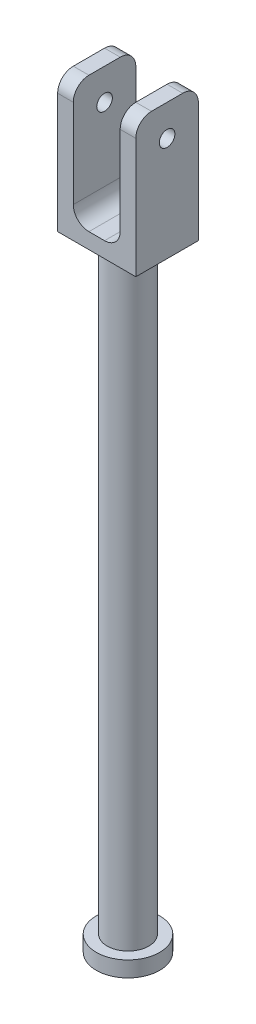
SolidWorks part; units mm, degrees
ref_plane "Front Plane" through (0, 0, 0) normal (0, 0, 1) x (1, 0, 0)
ref_plane "Top Plane" through (0, 0, 0) normal (0, 1, 0) x (1, 0, 0)
ref_plane "Right Plane" through (0, 0, 0) normal (1, 0, 0) x (0, 0, -1)
other "Configuration Table"
sketch "Sketch1" plane through (0, 0, 0) normal (0, 0, 1) x (1, 0, 0)
  line L0 (0, 26) -> (0, 0)
  line L1 (0, 0) -> (15, 0)
  line L2 (15, 0) -> (15, 26)
  line L3 (15, 26) -> (12, 26)
  line L4 (12, 26) -> (12, 3)
  line L5 (12, 3) -> (3, 3)
  line L6 (3, 3) -> (3, 26)
  line L7 (3, 26) -> (0, 26)
  dimension "D1" = 9
  dimension "D2" = 15
  dimension "D3" = 3
  dimension "D4" = 23
  dimension "D5" = 3
  dimension "D6" = 23
extrude "Boss-Extrude1" add sketch "Sketch1" along normal blind 12
fillet "Fillet1" radius 3 4 edges at (1.5, 26, 0) (13.5, 26, 0) (13.5, 26, 12) (1.5, 26, 12)
fillet "Fillet2" radius 3 2 edges at (12, 3, 6) (3, 3, 6)
sketch "Sketch2" plane through (15, 0, 0) normal (1, 0, 0) x (0, 0, -1)
  line L0 (-12, 0) -> (-12, 23) construction
  line L2 (-12, 0) -> (0, 0) construction
  circle A0 centre (-6, 20) radius 1.5
  dimension "D1" = 6
  dimension "D2" = 3
  dimension "D3" = 20
extrude "Cut-Extrude1" cut sketch "Sketch2" against normal through all
sketch "Sketch3" plane through (0, 0, 0) normal (0, -1, 0) x (-1, 0, 0)
  line L0 (0, -12) -> (-15, -12) construction
  circle A0 centre (-7.5, -6) radius 4
  dimension "D1" = 8
  dimension "D2" = 6
extrude "Boss-Extrude2" add sketch "Sketch3" along normal blind 116
sketch "Sketch4" plane through (0, -116, 0) normal (0, -1, 0) x (-1, 0, 0)
  circle A0 centre (-7.5, -6) radius 6.0817
extrude "Boss-Extrude3" add sketch "Sketch4" along normal blind 3
